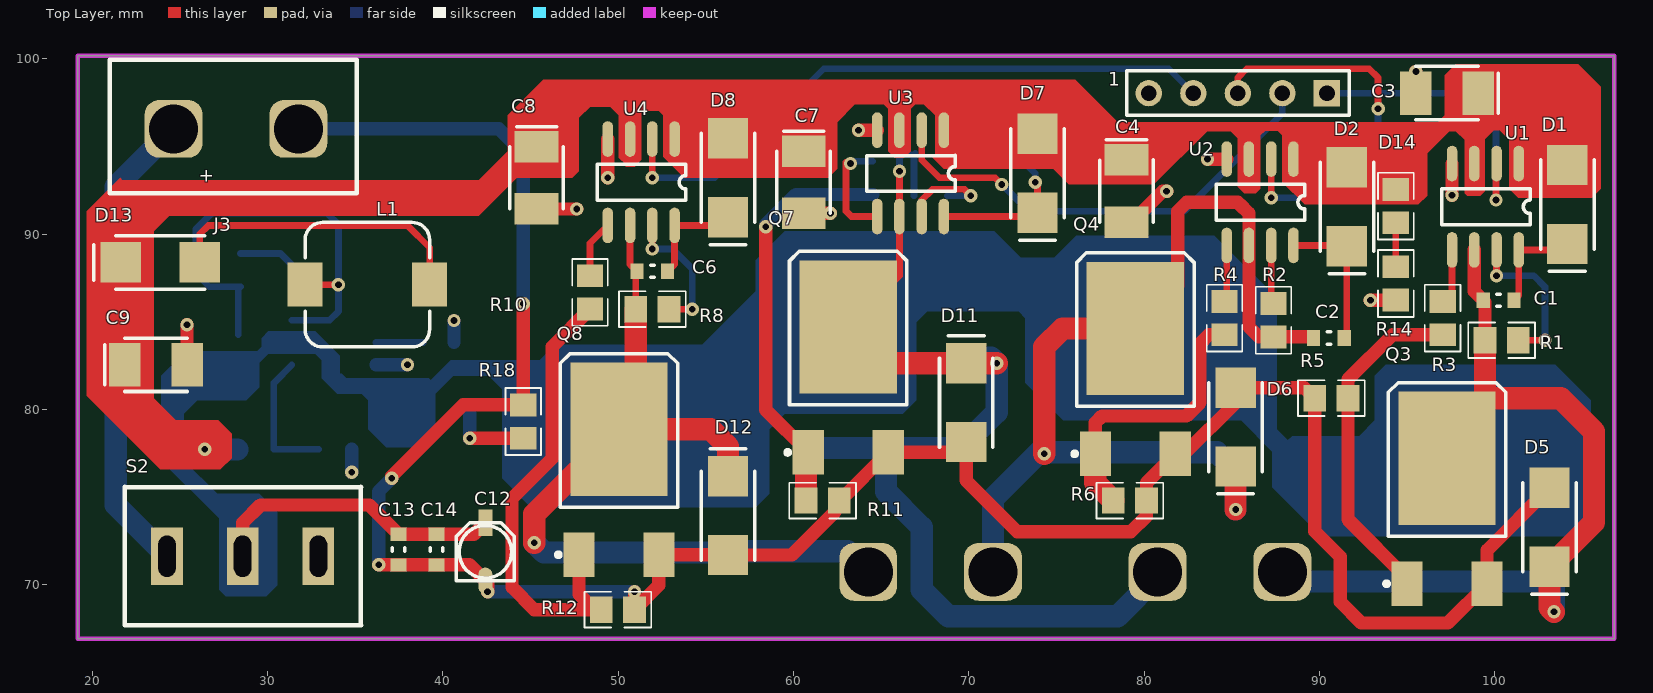
[diagram p0: Top Layer view]
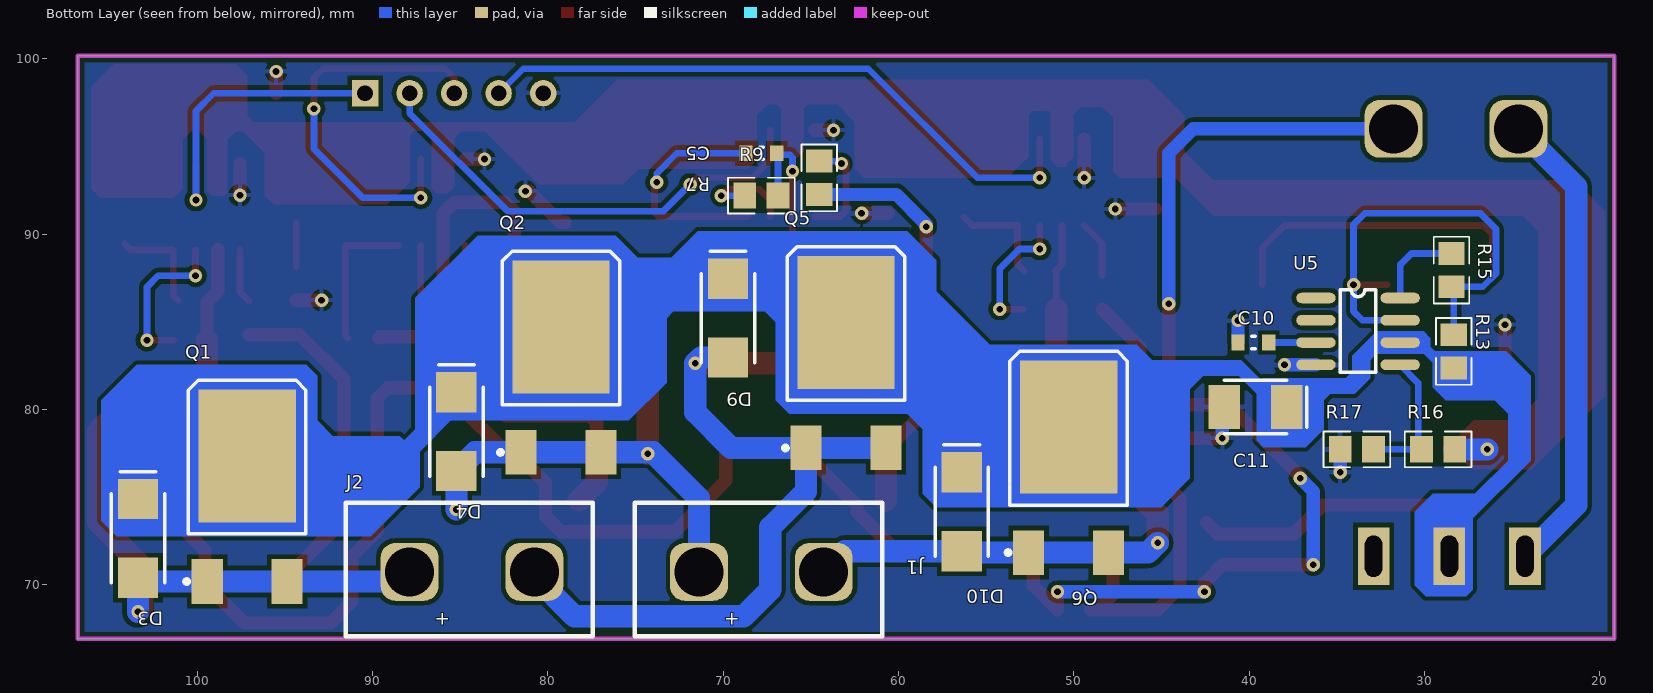
[diagram p1: Bottom Layer view, seen from below]
# Altium PCB MISC82071.PcbDoc
Units mm, origin at the board's own origin, x right, y up, seen from the top; angles counter-clockwise.
Board outline 87.63 x 33.24 mm, 2 copper layers (Top Layer, Bottom Layer); 65 components, 35 nets, 172 pads, 40 vias.

## Layer stack, top to bottom (the 12.6 mil dielectric is the usual default, probably not edited)
Top Solder: solder mask 0.0102, Solder Resist, Dk 3.5
Top Layer: signal copper 0.0356
Dielectric 1: dielectric 0.32, FR-4, Dk 4.8
Bottom Layer: signal copper 0.0356
Bottom Solder: solder mask 0.0102, Solder Resist, Dk 3.5

## Board outline
19.177,66.929 19.177,100.168 106.807,100.168 106.807,66.929

## Design rules (kind name [scope] priority, off if disabled: settings)
Clearance [All] p1: gap=0.254
Height [All] p1: minheight=0 maxheight=100 prefheight=12.7
HoleSize [All] p1: absolutevalues=TRUE maxlimit=254 minlimit=0.025 maxpercent=80.000 minpercent=20.000
MinimumSolderMaskSliver [All] p1: minsoldermaskwidth=0
PolygonConnect [All] p1: connectstyle=Relief reliefconductorwidth=0.254 reliefentries=4 polygonreliefangle="90 Angle" airgapwidth=0.254
RoutingVias [All] p1: holewidth=0.711 width=1.27 viastyle="Through Hole" minholewidth=0.711 minwidth=1.27 maxholewidth=0.711 maxwidth=1.27
SilkToSilkClearance [All] p1: silktosilkclearance=0
SilkToSolderMaskClearance [IsPad] p1: minsilkscreentomaskgap=0 clearancetoexposedcopper=TRUE
SolderMaskExpansion [All] p1: expansion=0.102
Width [All] p1: maxlimit=2.032 minlimit=0.254 preferedwidth=0.254
25 further rules are at their usual default settings.

## Components (designator, comment, footprint, x,y, rotation, side; value= is the part's Value field where it differs from the comment)
1 "Header 5" HDR1X5 90.424,98.044 r180 top
C1 "Cap" my0603 100.217,86.233 r180 top
C2 "Cap" my0603 90.537,84.074 r180 top
C3 "Cap Pol" CAP-3528 97.282,98.044 r180 top
C4 "Cap Pol" CAP-3528 78.994,92.456 r270 top
C5 "Cap" my0603 67.818,94.615 r180 bottom
C6 "Cap" my0603 51.943,87.884 r180 top
C7 "Cap Pol" CAP-3528 60.579,92.964 r270 top
C8 "Cap Pol" CAP-3528 45.339,93.218 r270 top
C9 "Cap Pol" CAP-3528 23.622,82.55 r0 top
C10 "Cap" my0603 39.751,83.82 r180 bottom
C11 "Cap Pol" CAP-3528 39.624,80.137 r0 bottom
C12 "Cap Pol" "CM A(3*5.4)" 42.418,71.882 r90 top
C13 "Cap" my0603 37.465,72.009 r90 top
C14 "Cap" my0603 39.624,72.009 r90 top
D1 "D-Schottky" DIODE-SMA 104.14,91.694 r270 top
D2 "D-Schottky" DIODE-SMA 91.567,91.567 r270 top
D3 "D-Schottky" DIODE-SMA 103.378,72.644 r90 bottom
D4 "D-Schottky" DIODE-SMA 85.217,78.74 r90 bottom
D5 "D-Schottky" DIODE-SMA 103.124,73.279 r270 top
D6 "D-Schottky" DIODE-SMA 85.217,78.994 r270 top
D7 "D-Schottky" DIODE-SMA 73.914,93.472 r270 top
D8 "D-Schottky" DIODE-SMA 56.261,93.218 r270 top
D9 "D-Schottky" DIODE-SMA 69.723,85.217 r90 bottom
D10 "D-Schottky" DIODE-SMA 56.388,74.168 r90 bottom
D11 "D-Schottky" DIODE-SMA 69.85,80.391 r90 top
D12 "D-Schottky" DIODE-SMA 56.261,73.95 r90 top
D13 "D-Schottky" DIODE-SMA 23.876,88.392 r180 top
D14 "LED0" 0805 94.361,91.606 r270 top
J1 "Pin2" "PCBComponent_1 - duplicate" 68.199,71.374 r270 bottom
J2 "Pin2" "PCBComponent_1 - duplicate" 84.709,71.374 r270 bottom
J3 "Pin2" "PCBComponent_1 - duplicate" 27.813,96.647 r270 top
L1 "Inductor" L-SMD-7 35.687,87.122 r180 top
Q1 "IR7843" LR7843 97.155,73.787 r270 bottom
Q2 "IR7843" LR7843 79.248,81.153 r270 bottom
Q3 "IR7843" LR7843 97.282,73.66 r270 top
Q4 "IR7843" LR7843 79.496,81.07 r270 top
Q5 "IR7843" LR7843 62.992,81.407 r270 bottom
Q6 "IR7843" LR7843 50.292,75.438 r270 bottom
Q7 "IR7843" LR7843 63.119,81.153 r270 top
Q8 "IR7843" LR7843 50.038,75.311 r270 top
R1 "Res1" 0805 100.396,83.947 r180 top
R2 "Res1" 0805 87.376,85.09 r270 top
R3 "Res1" 0805 97.028,85.217 r270 top
R4 "Res1" 0805 84.582,85.217 r270 top
R5 "Res1" 0805 90.678,80.645 r0 top
R6 "Res1" 0805 79.182,74.803 r180 top
R7 "Res1" 0805 67.818,92.202 r180 bottom
R8 "Res1" 0805 51.943,85.725 r180 top
R9 "Res1" 0805 64.516,93.218 r270 bottom
R10 "Res1" 0805 48.387,86.68 r270 top
R11 "Res1" 0805 61.661,74.803 r180 top
R12 "Res1" 0805 49.977,68.58 r180 top
R13 "Res1" 0805 28.321,83.312 r270 bottom
R14 "Res1" 0805 94.361,87.188 r270 top
R15 "Res1" 0805 28.448,87.95 r270 bottom
R16 "Res1" 0805 29.21,77.724 r0 bottom
R17 "Res1" 0805 33.848,77.724 r0 bottom
R18 "Res1" 0805 44.577,79.314 r270 top
S2 "SW-SPST" SWITCH 21.844,67.691 r0 top
U1 "IR2104S" IR2104 99.469,91.567 r270 top
U2 "IR2104S" IR2104 86.614,91.821 r270 top
U3 "IR2104S" IR2104 66.675,93.472 r270 top
U4 "IR2104S" IR2104 51.308,92.964 r270 top
U5 "MC34063" MC34063 33.782,84.455 r180 bottom

## Footprints (in the part's own frame and the unit in brackets; to place one, negate y for a bottom-side part, rotate by r counter-clockwise, add the part's x,y. Pads: shape width x height; smd on the part's side, far side on the other; paste and mask are expansions set on the pad)
0805 [mm]
  rect 1.3x1.5 smd: 1(-0.95,0) 2(0.95,0)
  silkscreen extent -1.91,-1.02 1.91,1.02, body extent -1.14,-0.51 1.14,0.51, height 1
CAP-3528 [mm]
  rect 1.8x2.5 smd: 1(-1.778,0) 2(1.778,0)
  silkscreen extent -2.92,-1.52 1.78,1.52, body extent -1.91,-1.4 1.91,1.4, height 1.1
"CM A(3*5.4)" [mm] "贴片电解电容，直径3mm，高5.4mm"
  rect 1.5x0.8 smd: 1(1.651,0)
  oval 1.5x0.8 smd: 2(-1.65,0)
  silkscreen extent -1.65,-1.65 1.65,1.65, body extent -1.9,-1.65 1.9,1.65, height 5.4
DIODE-SMA [mm]
  rect 2.3x2.3 smd: 1(-2.25,0) 2(2.25,0)
  silkscreen extent -2.54,-1.52 3.81,1.52, body extent -2.92,-1.4 2.92,1.4, height 3
HDR1X5 [mm]
  rect 1.5x1.5 hole 0.9: 1(0,0)
  round 1.5 hole 0.9: 2(2.54,0) 3(5.08,0) 4(7.62,0) 5(10.16,0)
  silkscreen extent -1.27,-1.27 11.43,1.27
IR2104 [mil]
  oval 80x23.62 smd: 1(-97,75) 2(-97,25) 3(-97,-25) 4(-97,-75) 5(97,-75) 6(97,-25) 7(97,25) 8(97,75)
  silkscreen extent -40,-98 40,100, body extent -118,-97 118,96, height 61
L-SMD-7 [mm]
  rect 2x2.5 smd: 1(-3.556,0) 2(3.556,0)
  silkscreen extent -3.56,-3.56 3.56,3.56, body extent -3.56,-3.56 3.56,3.56, height 4
LR7843 [mm]
  rect 2.54x1.778 smd: 1(3.6,-2.28) 3(3.6,2.28)
  rect 7.6x5.55 smd: 2(-3.556,0)
  silkscreen extent -7.87,-3.58 3.72,3.35, body extent -6.44,-3.32 3.5,3.22, height 2.39
MC34063 [mm]
  oval 2.25x0.6 smd: 1(-2.4,1.905) 2(-2.4,0.635) 3(-2.4,-0.635) 4(-2.4,-1.905) 5(2.4,-1.905) 6(2.4,-0.635) 7(2.4,0.635) 8(2.4,1.905)
  silkscreen extent -1.02,-2.34 1.02,2.37, body extent -2.99,-2.46 3,2.44, height 1.55
my0603 [mm]
  rect 0.75x0.9 smd: 1(-0.875,0) 2(0.875,0)
  silkscreen extent -0.1,-0.35 0.1,0.35, body extent -0.8,-0.4 0.8,0.4, height 0.5
"PCBComponent_1 - duplicate" [mil]
  rrect50% 130x130 hole 110: 1(25,-125) 2(25,155)
  silkscreen extent -130,-269 170,286
SWITCH [mm]
  rect 1.8x3.3 hole 1 slot 2.35 at 90 deg: 1(2.413,3.937) 2(6.731,3.937)
  rect 1.8x3.3 / inner rect 0x0 / far side rect 1.8x3.3 hole 1 slot 2.35 at 90 deg mask+0.102: 3(11.049,3.937)
  silkscreen extent 0,0 13.5,7.9, body extent 0.38,0.51 13.1,7.37, height 28.55

## Part data
1: "Header, 5-Pin"
C1 C2 C5 C6 C10 C13 C14: "Non-polarized capacitor"
C3 C4 C7 C8 C9 C11 C12: "Polarized electrolytic capacitor"
D1 D2 D3 D4 D5 D6 D7 D8 D9 D10 D11 D12 D13: "Schottky diode"
D14: "LED"
Q1 Q2 Q3 Q4 Q5 Q6 Q7 Q8: library part NMOS, "N-Channel Power MOSFET"
R1 R2 R3 R4 R5 R6 R7 R8 R9 R10 R11 R12 R13 R14 R15 R16 R17 R18: "Chip resistor"
S2: "Single-Pole, Single-Throw Switch"
U1 U2 U3 U4: library part IR2104

## Via types
v1: diameter 0.762, hole 0.381, Top Layer to Bottom Layer, 40 vias

## Nets (pads, with @x,y where several pads share a name; then routed paths per layer and width w, separated by ;. In a path a pad name is that pad's centre, name@x,y a point inside that pad or via, vN(x,y) a via of type N, cw(c..) or ccw(c..) an arc to the next point about the centre after c; other vN are vias at no path point)
+12: C3.1 C4.1 C7.1 C8.1 C9.1 D1.1 D2.1 D7.1 D8.1 D13.2 D14.1 R16.1 U1.1 U1.3 U2.1 U2.3 U3.1 U3.3 U4.1 U4.3 | length 1.8
  Bottom Layer w1.27: v1(26.416,77.724) R16.1
BGND: C12.2 C13.1 C14.1 D5.1 D6.1 D11.1 D12.1 J3.2 Q3.3 Q4.3 Q7.3 Q8.3 R5.1 R6.1 R11.1 R12.1 R18.1 | length 140.5
  Top Layer w0.762: v1(36.336,71.134) C13.1 C14.1 41.516,71.134 C12.2 42.545,70.105 v1(42.545,69.596) ; v1(37.084,76.073) 37.084,76.2 41.148,80.264 R18.1 v1(44.577,86.04) ; v1(50.927,69.596) R12.1 52.318,69.971 Q8.3 56.25,71.711 D12.1 59.906,71.7 62.366,74.159 62.366,74.558 R11.1 62.649,74.803 Q7.3 69.262,77.553 D11.1 69.85,75.946 72.771,73.025 79.242,73.025 80.132,73.915 R6.1 80.132,75.826 Q4.3 82.296,77.47 85.217,80.391 D6.1 89.129,81.244 R5.1 89.728,73.053 91.186,71.595 91.186,69.022 92.39,67.818 97.32,67.818 Q3.3 99.562,71.967 D5.1
  Bottom Layer w0.762: J3.2 43.18,96.012 44.577,94.615 v1(44.577,86.04) ; v1(36.336,71.134) 36.336,75.325 v1(37.084,76.073) ; v1(42.545,69.596) v1(50.927,69.596)
GND: 1.5 C3.2 C4.2 C7.2 C8.2 C9.2 C10.1 C11.2 R14.2 R17.2 R18.2 U1.4 U2.4 U3.4 U4.4 U5.4 | length 27.2
  Top Layer w0.762: C9.2 v1(25.4,84.836) ; v1(41.524,78.364) R18.2 ; C8.2 v1(47.625,91.44) ; v1(49.403,93.218) U4.4 ; C7.2 v1(62.103,91.186) ; v1(63.703,95.936) U3.4 ; C4.2 79.293,90.678 81.071,92.456 v1(81.28,92.456) ; v1(83.617,94.285) U2.4 ; v1(92.908,86.238) R14.2 ; C3.2 v1(95.504,99.279) ; v1(97.564,92.23) U1.4
  Bottom Layer w0.762: v1(34.798,76.418) R17.2 ; U5.4 v1(37.973,82.55) ; C10.1 v1(40.626,85.076) ; C11.2 41.524,80.015 v1(41.524,78.364)
MOTOR1: C1.2 D3.1 D5.2 J2.1 Q1.1 Q1.3 Q3.2 R1.2 U1.6 | length 44.9
  Top Layer w0.762: U1.6 98.834,86.741 C1.2 99.446,86.129 R1.2
  Top Layer w1.27: R1.2 99.446,80.645 103.759,80.645 105.664,78.74 105.664,73.569 D5.2 103.124,68.707 v1(103.378,68.453)
  Bottom Layer w1.27: J2.1 88.436,70.187 Q1.3 Q1.1 103.171,70.187 D3.1 v1(103.378,68.453)
MOTOR2: C5.2 D9.1 D11.2 J2.2 Q5.1 Q5.3 Q7.2 R7.2 U3.6 | length 64.3
  Top Layer w0.381: Q7.2 66.04,87.63 U3.6 v1(66.04,93.599)
  Top Layer w1.27: Q7.2 65.187,82.641 D11.2 v1(71.592,82.641)
  Bottom Layer w0.381: v1(66.04,93.599) 66.04,94.361 66.219,94.54 C5.2@66.868,94.54 ; R7.2 C5.2@66.868,94.54 ; C5.2 C5.2@66.868,94.54
  Bottom Layer w1.27: Q5.3 Q5.1 ; D9.1 71.266,82.967 v1(71.592,82.641) 71.592,79.847 69.552,77.807 Q5.1 ; J2.2 80.772,70.485 78.486,68.199 68.834,68.199 67.31,69.723 67.31,73.279 65.272,75.317 Q5.1
MOTOR3: C2.2 D4.1 D6.2 J1.1 Q2.1 Q2.3 Q4.2 R2.2 U2.6 | length 58.6
  Top Layer w0.762: Q4.2 81.915,87.045 81.915,91.313 82.423,91.821 85.335,91.821 85.462,91.694 85.471,91.694 85.979,91.186 U2.6 85.979,84.709 86.548,84.14 R2.2 89.596,84.14 C2.2
  Top Layer w1.27: v1(74.295,77.47) 74.295,83.566 75.355,84.626 Q4.2 ; v1(85.217,74.295) D6.2
  Bottom Layer w1.27: J1.1 71.374,74.93 73.997,77.553 Q2.3 Q2.1 84.154,77.553 D4.1 v1(85.217,74.295)
MOTOR4: C6.2 D10.1 D12.2 J1.2 Q6.1 Q6.3 Q8.2 R8.2 U4.6 | length 48.8
  Top Layer w0.381: U4.6 50.673,88.279 C6.2 50.993,87.809 R8.2
  Top Layer w1.27: v1(45.212,72.39) 45.212,74.041 Q8.2 ; R8.2 50.993,79.822 Q8.2 ; D12.2 56.261,77.887 55.281,78.867 Q8.2
  Bottom Layer w1.27: v1(45.212,72.39) 45.764,71.838 Q6.3 Q6.1 56.308,71.838 D10.1 63.083,71.918 J1.2
NetC1_1: C1.1 D1.2 U1.8 | length 5.9
  Top Layer w0.381: C1.1 101.374,86.515 U1.8 103.799,89.103 D1.2
NetC2_1: C2.1 D2.2 U2.8 | length 8.4
  Top Layer w0.381: U2.8 91.527,89.357 D2.2 91.567,84.229 C2.1
NetC5_1: C5.1 D7.2 U3.8 | length 13.3
  Top Layer w0.381: U3.8 73.7,91.008 D7.2 73.914,92.837 v1(73.787,92.964)
  Bottom Layer w0.381: C5.1 72.644,94.615 73.787,93.472 v1(73.787,92.964)
NetC6_1: C6.1 D8.2 U4.8 | length 6
  Top Layer w0.381: C6.1 53.213,88.279 U4.8 55.793,90.5 D8.2
NetC10_2: C10.2 U5.3 | length 2.7
  Bottom Layer w0.381: U5.3 C10.2
NetD13_1: D13.1 L1.1 | length 17.6
  Top Layer w0.381: D13.1 26.126,90.007 26.619,90.5 37.973,90.5 39.243,89.23 L1.1
NetD14_2: D14.2 R14.1 | length 2.5
  Top Layer w0.381: R14.1 D14.2
NetL1_2: L1.2 R13.1 R15.2 U5.7 | length 26.7
  Top Layer w0.381: L1.2 v1(34.036,87.122)
  Bottom Layer w0.381: R13.1 28.321,86.873 R15.2 26.665,87 25.908,87.757 25.908,90.297 26.797,91.186 33.401,91.186 34.036,90.551 v1(34.036,87.122) 34.036,85.598 33.528,85.09 U5.7
NetQ3_1: Q3.1 R3.2 R5.2 | length 19.5
  Top Layer w0.762: Q3.1 95.002,70.352 91.628,73.726 R5.2 91.628,81.722 94.173,84.267 R3.2
NetQ4_1: Q4.1 R4.2 R6.2 | length 16.3
  Top Layer w0.762: Q4.1 77.216,79.248 77.597,79.629 82.416,79.629 83.185,80.398 83.185,83.759 83.693,84.267 R4.2
  Top Layer w1.27: Q4.1 77.216,75.819 R6.2
NetQ7_1: Q7.1 R9.2 R11.2 | length 23.6
  Top Layer w0.762: v1@58.42,90.402 58.42,79.972 Q7.1
  Top Layer w1.27: R11.2 60.711,77.425 Q7.1
  Bottom Layer w0.762: v1(58.42,90.424) 58.42,90.551 60.137,92.268 R9.2
NetQ8_1: Q8.1 R10.2 R12.2 | length 26.8
  Top Layer w0.762: Q8.1 47.758,69.463 R12.2@48.641,68.58 ; R10.2 46.228,83.571 46.228,77.216 43.942,74.93 43.942,69.85 45.212,68.58 R12.2@48.641,68.58 ; R12.2 R12.2@48.641,68.58
NetR1_1: R1.1 U1.7 | length 9.2
  Top Layer w0.381: v1(100.104,87.63) U1.7 ; R1.1 v1(102.87,83.947) v1@102.997,83.947
  Bottom Layer w0.381: v1(100.104,87.63) 102.235,87.63 102.87,86.995 v1(102.87,83.947)
NetR2_1: R2.1 U2.7 | length 3.4
  Top Layer w0.381: U2.7 87.249,86.167 R2.1
NetR3_1: R3.1 U1.5 | length 3.2
  Top Layer w0.381: R3.1 97.564,86.703 U1.5
NetR4_1: R4.1 U2.5 | length 3.4
  Top Layer w0.381: U2.5 84.709,86.487 R4.1@85.09,86.106
NetR7_1: R7.1 U3.7 | length 5.5
  Top Layer w0.381: U3.7 67.31,91.948 67.918,92.556 69.75,92.556 v1(70.104,92.202)
  Bottom Layer w0.381: R7.1 v1(70.104,92.202)
NetR8_1: R8.1 U4.7 | length 7.7
  Top Layer w0.381: v1(51.943,89.154) U4.7 ; R8.1 v1(54.229,85.725)
  Bottom Layer w0.381: v1(51.943,89.154) 53.086,89.154 54.229,88.011 v1(54.229,85.725)
NetR9_1: R9.1 U3.5 | length 6.4
  Top Layer w0.381: v1@62.992,94.107 v1@62.992,93.777 ; v1(63.246,94.031) v1@62.992,93.777 ; U3.5 63.297,91.008 62.992,91.313 v1@62.992,93.777
  Bottom Layer w0.381: v1(63.246,94.031) 63.383,94.168 R9.1
NetR10_1: R10.1 U4.5 | length 3.3
  Top Layer w0.381: R10.1 48.387,89.484 U4.5
NetR15_1: R15.1 U5.8 | length 5.1
  Bottom Layer w0.381: R15.1 30.734,88.9 31.382,88.252 U5.8
NetR16_2: R16.2 R17.1 U5.5 | length 7.8
  Bottom Layer w0.381: U5.5 30.353,81.521 30.353,77.724 R17.1
PWM1_OUT: 1.1 U1.2 | length 17.2
  Top Layer w0.381: v1(100.076,91.948) 100.076,94.003 U1.2
  Bottom Layer w0.381: 1.1 99.06,98.044 100.076,97.028 v1(100.076,91.948)
PWM2_OUT: 1.2 U3.2 | length 26.9
  Top Layer w0.381: U3.2 67.31,94.234 68.326,93.218 71.501,93.218 v1(71.882,92.837)
  Bottom Layer w0.381: v1(71.882,92.837) 73.406,91.313 82.296,91.313 87.884,96.901 1.2
PWM3_OUT: 1.3 U2.2 | length 22.8
  Top Layer w0.381: 1.3 85.344,98.933 85.852,99.441 92.837,99.441 93.345,98.933 v1(93.345,97.155) ; v1(87.249,92.075) U2.2
  Bottom Layer w0.381: v1(87.249,92.075) 90.551,92.075 93.345,94.869 v1(93.345,97.155)
PWM4_OUT: 1.4 U4.2 | length 36.2
  Top Layer w0.381: v1(51.943,93.218) U4.2
  Bottom Layer w0.381: v1(51.943,93.218) 55.499,93.218 61.722,99.441 81.407,99.441 1.4
VCC_BATTERY: J3.1 S2.1 | length 27
  Bottom Layer w1.27: S2.1 21.336,74.549 21.336,92.71 J3.1
VCC_MOTOR: C11.1 C12.1 C13.2 C14.2 D3.2 D4.2 D9.2 D10.2 Q1.2 Q2.2 Q5.2 Q6.2 R13.2 S2.2 U5.6 | length 17.1
  Top Layer w0.762: S2.2 28.575,73.533 29.591,74.549 35.8,74.549 C13.2 C14.2 41.769,72.884 C12.1
pads on no net: S2.3 U5.1 U5.2

## Polygon pours and split planes (outlines as drawn)
GND on Bottom Layer "D" (solid, remove dead copper, pour order 16): 17.399,102.362 18.161,101.6 108.585,101.6 108.585,66.421 108.458,66.294 108.077,65.913 15.748,65.913

## Keep-outs
Keep-Out Layer:
  the board outline again, w0.254

## Other copper
Top Layer:
  region net +12: 27.305,76.581 23.876,76.581 19.685,80.772 19.685,91.313 21.59,93.218 21.717,93.091 42.037,93.091 43.688,94.742 43.688,96.774 45.72,98.806 76.073,98.806 78.486,96.393 96.774,96.393 97.155,96.774 97.155,99.06 97.79,99.695 104.775,99.695 106.045,98.425 106.045,92.583 105.537,92.075 101.346,92.075 100.838,92.583 100.838,95.391 100.293,95.936 97.496,95.936 99.949,95.936 99.441,95.428 99.441,92.456 99.187,92.202 98.425,92.202 98.298,92.329 98.298,95.377 97.79,95.885 97.409,95.885 96.139,94.615 96.139,92.202 95.631,91.694 89.154,91.694 87.884,92.964 87.884,95.631 87.616,95.899 86.868,95.899 86.868,95.885 86.614,95.631 86.614,92.583 86.36,92.329 85.725,92.329 85.344,92.71 85.344,95.468 84.927,95.885 83.602,95.885 80.554,92.837 75.692,92.837 74.803,93.726 68.58,93.726 67.945,94.361 68.072,94.488 68.072,96.774 67.437,97.409 66.929,97.409 66.675,97.155 66.675,94.742 66.294,94.361 65.786,94.361 65.405,94.742 65.405,96.266 65.399,97.161 65.151,97.409 63.5,97.409 62.484,96.393 62.484,93.726 61.976,93.218 53.772,93.218 52.578,94.412 52.578,96.774 52.324,97.028 51.435,97.028 51.308,96.901 51.308,94.234 50.927,93.853 50.419,93.853 50.419,93.98 50.038,94.361 50.038,96.774 49.53,97.282 48.393,97.282 47.752,96.641 47.752,93.599 47.371,93.218 44.196,93.218 42.037,91.059 24.384,91.059 23.495,90.17 23.495,80.645 24.765,79.375 27.178,79.375 27.94,78.613 27.94,77.216
Bottom Layer:
  region net VCC_MOTOR: 27.241,69.723 27.241,73.787 23.939,77.089 23.939,81.915 25.336,83.312 29.4,83.312 29.654,83.566 29.654,84.074 30.035,84.455 32.703,84.455 34.099,83.058 34.099,82.042 34.227,82.042 34.48,81.788 39.179,81.788 39.306,81.661 40.45,82.804 45.529,82.804 46.419,83.693 54.8,83.693 57.848,86.741 57.848,88.519 59.499,90.17 71.438,90.17 72.962,88.646 74.867,88.646 76.136,89.916 84.01,89.916 87.566,86.36 87.566,78.867 88.201,78.232 88.456,78.486 92.266,78.486 93.154,79.375 93.154,81.915 93.789,82.55 103.441,82.55 105.474,80.518 105.474,73.66 104.584,72.771 90.106,72.771 87.312,75.565 87.312,77.597 85.534,79.375 75.374,79.375 73.215,81.534 73.215,85.217 72.834,85.598 67.627,85.598 66.992,84.963 66.992,80.518 66.23,79.756 59.499,79.756 58.61,78.867 58.61,75.184 57.848,74.422 45.021,74.422 43.37,76.073 43.37,81.153 42.608,81.915 40.576,81.915 39.56,80.899 39.56,78.232 39.179,77.851 36.767,77.851 35.75,78.867 35.75,80.518 35.369,80.899 33.972,80.899 33.084,81.788 33.084,82.804 32.703,83.185 30.035,83.185 29.527,82.677 29.527,81.28 28.765,80.518 25.971,80.518 25.209,79.756 25.209,77.089 27.114,75.184 29.527,75.184 30.543,74.168 30.543,69.977 29.909,69.342 27.622,69.342